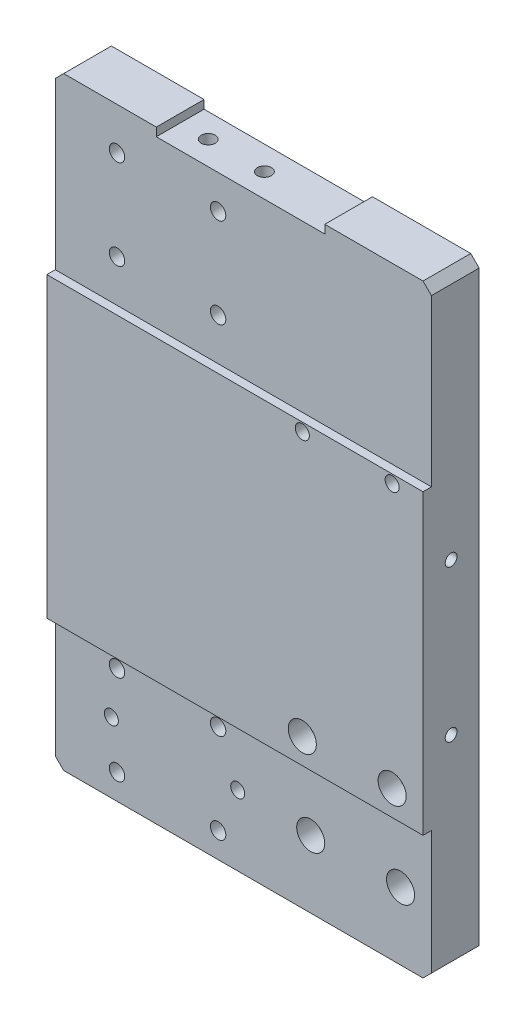
SolidWorks part; units mm, degrees
material "Q235-A"
ref_plane "Front Plane" through (0, 0, 0) normal (0, 0, 1) x (1, 0, 0)
ref_plane "Top Plane" through (0, 0, 0) normal (0, 1, 0) x (1, 0, 0)
ref_plane "Right Plane" through (0, 0, 0) normal (1, 0, 0) x (0, 0, -1)
sketch "Sketch1" plane through (0, 3.6076, 0) normal (1, 0, 0) x (0, 0, -1)
  line L0 (-22.9317, -128.8807) -> (-22.9317, -175.8807)
  line L1 (-22.9317, 39.1193) -> (-5.9317, 39.1193)
  line L2 (-22.9317, 39.1193) -> (-22.9317, -22.8807)
  line L3 (-22.9317, -175.8807) -> (-5.9317, -175.8807)
  line L4 (-5.9317, 39.1193) -> (-5.9317, -175.8807)
  line L5 (-22.9317, -128.8807) -> (-25.9317, -128.8807)
  line L7 (-22.9317, -22.8807) -> (-25.9317, -22.8807)
  line L8 (-25.9317, -128.8807) -> (-25.9317, -22.8807)
  dimension "D1" = 17
  dimension "D2" = 215
  dimension "D3" = 3
  dimension "D4" = 106
  dimension "D5" = 47
extrude "Boss-Extrude1" add sketch "Sketch1" along normal blind 134
sketch "Sketch2" plane through (0, 3.6076, 22.9317) normal (0, 0, 1) x (1, 0, 0)
  line L0 (134, 39.1193) -> (0, 39.1193) construction
  line L1 (36, 39.1193) -> (96, 39.1193)
  line L2 (36, 39.1193) -> (36, 36.1193)
  line L3 (36, 36.1193) -> (96, 36.1193)
  line L4 (96, 39.1193) -> (96, 36.1193)
  dimension "D1" = 60
  dimension "D2" = 3
  dimension "D3" = 38
extrude "Cut-Extrude1" cut sketch "Sketch2" against normal blind 134
chamfer "Chamfer1" distance 3 angle 45 4 edges at (0, -172.2731, 14.4317) (134, -172.2731, 14.4317) (134, 42.7269, 14.4317) (0, 42.7269, 14.4317)
sketch "Sketch3" plane through (134, 3.6076, 0) normal (1, 0, 0) x (0, 0, -1)
  line L0 (-15.9317, -48.8807) -> (-15.9317, -102.8807)
  line L1 (-5.9317, -175.8807) -> (-22.9317, -175.8807) construction
  line L2 (-5.9317, -172.8807) -> (-5.9317, 36.1193) construction
  dimension "D1" = 54
  dimension "D2" = 73
  dimension "D3" = 10
sketch "Sketch6" plane through (0, 3.6076, 0) normal (-1, 0, 0) x (0, 0, 1)
  line L0 (15.9317, -48.8807) -> (15.9317, -102.8807) construction
  line L1 (15.9317, -48.8807) -> (15.9317, -102.8807)
hole_wizard "M5 Tapped Hole1" positions "Sketch4" profile "Sketch5" tap size "M5" standard "GB"
sketch "Sketch4" plane through (134, 0, 0) normal (1, 0, 0) x (0, 0, -1)
  point P0 (-15.9317, -45.2731)
  point P3 (-15.9317, -99.2731)
sketch "Sketch5" plane through (134, -45.2731, 15.9317) normal (0, 1, 0) x (0, 0, -1)
  line L0 (0, 0) -> (0, 10)
  line L1 (0, 10) -> (2.1, 8.7382)
  line L2 (2.1, 8.7382) -> (2.1, 0)
  line L5 (2.1, 0) -> (0, 0)
  line L10 (0, 10) -> (-2.1, 8.7382) construction
  line L11 (0, -6.35) -> (0, 107.95) construction
  dimension "螺纹孔钻头直径" = 4.2
  dimension "螺纹孔钻头深度" = 10
  dimension "导头角度" = 118
cosmetic thread "Cosmetic thread 1" parameters "D1"=8.7382, "D2"=5
cosmetic thread "Cosmetic thread 2" parameters "D1"=8.7382, "D2"=5
hole_wizard "M5 Tapped Hole2" positions "Sketch7" profile "Sketch8" tap size "M5" standard "GB"
sketch "Sketch7" plane through (0, 0, 0) normal (-1, 0, 0) x (0, 0, 1)
  point P0 (15.9317, -45.2731)
  point P3 (15.9317, -99.2731)
sketch "Sketch8" plane through (0, -45.2731, 15.9317) normal (0, 1, 0) x (0, 0, 1)
  line L0 (0, 0) -> (0, 10)
  line L1 (0, 10) -> (2.1, 8.7382)
  line L2 (2.1, 8.7382) -> (2.1, 0)
  line L5 (2.1, 0) -> (0, 0)
  line L10 (0, 10) -> (-2.1, 8.7382) construction
  line L11 (0, -6.35) -> (0, 107.95) construction
  dimension "螺纹孔钻头直径" = 4.2
  dimension "螺纹孔钻头深度" = 10
  dimension "导头角度" = 118
cosmetic thread "Cosmetic thread 3" parameters "D1"=8.7382, "D2"=5
cosmetic thread "Cosmetic thread 4" parameters "D1"=8.7382, "D2"=5
sketch "Sketch9" plane through (0, 39.7269, 0) normal (0, 1, 0) x (1, 0, 0)
  line L0 (66, -14.4317) -> (46, -14.4317)
  line L1 (36, -5.9317) -> (96, -5.9317) construction
  line L2 (36, -5.9317) -> (36, -22.9317) construction
  dimension "D1" = 20
  dimension "D2" = 8.5
  dimension "D3" = 10
hole_wizard "M6 Tapped Hole1" positions "Sketch10" profile "Sketch11" tap size "M6" standard "GB"
sketch "Sketch10" plane through (0, 39.7269, 0) normal (0, 1, 0) x (1, 0, 0)
  point P0 (66, -14.4317)
  point P3 (46, -14.4317)
sketch "Sketch11" plane through (66, 39.7269, 14.4317) normal (1, 0, 0) x (0, 0, 1)
  line L0 (0, 0) -> (0, 12)
  line L1 (0, 12) -> (2.5, 10.4978)
  line L2 (2.5, 10.4978) -> (2.5, 0)
  line L5 (2.5, 0) -> (0, 0)
  line L10 (0, 12) -> (-2.5, 10.4978) construction
  line L11 (0, -6.35) -> (0, 107.95) construction
  dimension "螺纹孔钻头直径" = 5
  dimension "螺纹孔钻头深度" = 12
  dimension "导头角度" = 118
cosmetic thread "Cosmetic thread 5" parameters "D1"=10.4978, "D2"=6
cosmetic thread "Cosmetic thread 6" parameters "D1"=10.4978, "D2"=6
sketch "Sketch12" plane through (0, 3.6076, 5.9317) normal (0, 0, -1) x (-1, 0, 0)
  line L0 (-131, -175.8807) -> (-3, -175.8807) construction
  line L1 (-58, 24.1193) -> (-22, 24.1193)
  line L2 (-58, 24.1193) -> (-58, -7.8807)
  line L3 (-58, -7.8807) -> (-22, -7.8807)
  line L4 (-22, 24.1193) -> (-22, -7.8807)
  line L5 (-58, -134.8807) -> (-22, -134.8807)
  line L6 (-58, -134.8807) -> (-58, -166.8807)
  line L7 (-58, -166.8807) -> (-22, -166.8807)
  line L8 (-22, -134.8807) -> (-22, -166.8807)
  line L9 (-123, -25.8807) -> (-91, -25.8807)
  line L10 (0, -172.8807) -> (0, 36.1193) construction
  dimension "D1" = 32
  dimension "D2" = 36
  dimension "D3" = 32
  dimension "D4" = 36
  dimension "D5" = 159
  dimension "D6" = 9
  dimension "D7" = 32
  dimension "D8" = 91
  dimension "D9" = 150
  dimension "D10" = 22
  dimension "D11" = 22
hole_wizard "M6 Tapped Hole2" positions "Sketch13" profile "Sketch14" tap size "M6" standard "GB" end condition through all
sketch "Sketch13" plane through (0, 0, 5.9317) normal (0, 0, -1) x (-1, 0, 0)
  point P0 (-123, -22.2731)
  point P3 (-91, -22.2731)
sketch "Sketch14" plane through (123, -22.2731, 5.9317) normal (1, 0, 0) x (0, 1, 0)
  line L0 (0, 0) -> (0, 20)
  line L1 (0, 20) -> (2.5, 20)
  line L2 (2.5, 20) -> (2.5, 0)
  line L5 (2.5, 0) -> (0, 0)
  line L11 (0, -6.35) -> (0, 107.95) construction
  dimension "通孔螺纹孔钻头直径" = 5
  dimension "通孔螺纹孔钻头深度" = 20
cosmetic thread "Cosmetic thread 7" parameters "D2"=6
cosmetic thread "Cosmetic thread 8" parameters "D2"=6
hole_wizard "Hole1" positions "Sketch15" profile "Sketch16" legacy end condition through all
sketch "Sketch15" plane through (0, 0, 5.9317) normal (0, 0, -1) x (-1, 0, 0)
  point P0 (-58, 27.7269)
  point P3 (-22, 27.7269)
  point P6 (-22, -4.2731)
  point P9 (-58, -4.2731)
  point P12 (-58, -131.2731)
  point P15 (-58, -163.2731)
  point P18 (-22, -163.2731)
  point P21 (-22, -131.2731)
sketch "Sketch16" plane through (58, 27.7269, 5.9317) normal (1, 0, 0) x (0, 1, 0)
  line L0 (0, 0) -> (0, 20)
  line L1 (0, 20) -> (2.75, 20)
  line L2 (2.75, 20) -> (2.75, 7)
  line L3 (2.75, 7) -> (5, 7)
  line L4 (5, 7) -> (5, 0)
  line L5 (5, 0) -> (0, 0)
  line L6 (0, 110) -> (0, -10) construction
  dimension "直径" = 5.5
  dimension "深度" = 20
  dimension "柱坑直径" = 10
  dimension "柱坑深度" = 7
sketch "Sketch17" plane through (0, 0, 5.9317) normal (0, 0, -1) x (-1, 0, 0)
  line L0 (-131, -172.2731) -> (-3, -172.2731) construction
  line L1 (-129, -172.2731) -> (-83, -172.2731)
  line L2 (-129, -172.2731) -> (-129, -77.2731)
  line L3 (-124, -72.2731) -> (-88, -72.2731)
  line L4 (-83, -172.2731) -> (-83, -77.2731)
  line L5 (0, -169.2731) -> (0, 39.7269) construction
  arc A0 (-83, -77.2731) -> (-88, -72.2731) centre (-88, -77.2731) ccw
  arc A1 (-129, -77.2731) -> (-124, -72.2731) centre (-124, -77.2731) cw
  point P12 (-129, -72.2731)
  dimension "D4" = 5
  dimension "D1" = 100
  dimension "D2" = 46
  dimension "D3" = 83
extrude "Cut-Extrude2" cut sketch "Sketch17" against normal blind 3
sketch "Sketch18" plane through (0, 0, 25.9317) normal (0, 0, 1) x (1, 0, 0)
  line L1 (91, -22.2731) -> (123, -22.2731)
  line L2 (91, -22.2731) -> (91, -116.2731)
  line L3 (91, -116.2731) -> (123, -116.2731)
  line L4 (123, -22.2731) -> (123, -116.2731)
  line L5 (91, -116.2731) -> (123, -116.2731)
  line L6 (91, -116.2731) -> (91, -148.2731)
  line L7 (91, -148.2731) -> (123, -148.2731)
  line L8 (123, -116.2731) -> (123, -148.2731)
  dimension "D1" = 32
  dimension "D2" = 94
  dimension "D3" = 32
hole_wizard "Hole2" positions "Sketch19" profile "Sketch20" legacy end condition through all
sketch "Sketch19" plane through (0, 0, 25.9317) normal (0, 0, 1) x (1, 0, 0)
  point P0 (91, -116.2731)
  point P3 (123, -116.2731)
sketch "Sketch20" plane through (91, -116.2731, 25.9317) normal (1, 0, 0) x (0, -1, 0)
  line L0 (0, 0) -> (0, 20)
  line L1 (0, 20) -> (2.75, 20)
  line L2 (2.75, 20) -> (2.75, 7)
  line L3 (2.75, 7) -> (5, 7)
  line L4 (5, 7) -> (5, 0)
  line L5 (5, 0) -> (0, 0)
  line L6 (0, 110) -> (0, -10) construction
  dimension "直径" = 5.5
  dimension "深度" = 20
  dimension "柱坑直径" = 10
  dimension "柱坑深度" = 7
hole_wizard "Hole3" positions "Sketch21" profile "Sketch22" legacy end condition through all
sketch "Sketch21" plane through (0, 0, 22.9317) normal (0, 0, 1) x (1, 0, 0)
  point P0 (91, -148.2731)
  point P3 (123, -148.2731)
sketch "Sketch22" plane through (91, -148.2731, 22.9317) normal (1, 0, 0) x (0, -1, 0)
  line L0 (0, 0) -> (0, 17)
  line L1 (0, 17) -> (2.75, 17)
  line L2 (2.75, 17) -> (2.75, 7)
  line L3 (2.75, 7) -> (5, 7)
  line L4 (5, 7) -> (5, 0)
  line L5 (5, 0) -> (0, 0)
  line L6 (0, 110) -> (0, -10) construction
  dimension "直径" = 5.5
  dimension "深度" = 17
  dimension "柱坑直径" = 10
  dimension "柱坑深度" = 7
sketch "Sketch23" plane through (0, 0, 22.9317) normal (0, 0, 1) x (1, 0, 0)
  line L0 (20, -147.2731) -> (65, -147.2731)
  line L1 (0, -125.2731) -> (0, -169.2731) construction
  line L2 (131, -172.2731) -> (3, -172.2731) construction
  dimension "D1" = 20
  dimension "D2" = 45
  dimension "D3" = 25
hole_wizard "M6 Tapped Hole3" positions "Sketch24" profile "Sketch25" tap size "M6" standard "GB" end condition through all
sketch "Sketch24" plane through (0, 0, 22.9317) normal (0, 0, 1) x (1, 0, 0)
  point P0 (20, -147.2731)
  point P3 (65, -147.2731)
sketch "Sketch25" plane through (20, -147.2731, 22.9317) normal (1, 0, 0) x (0, -1, 0)
  line L0 (0, 0) -> (0, 17)
  line L1 (0, 17) -> (2.5, 17)
  line L2 (2.5, 17) -> (2.5, 0)
  line L5 (2.5, 0) -> (0, 0)
  line L11 (0, -6.35) -> (0, 107.95) construction
  dimension "通孔螺纹孔钻头直径" = 5
  dimension "通孔螺纹孔钻头深度" = 17
cosmetic thread "Cosmetic thread 9" parameters "D2"=6
cosmetic thread "Cosmetic thread 10" parameters "D2"=6
